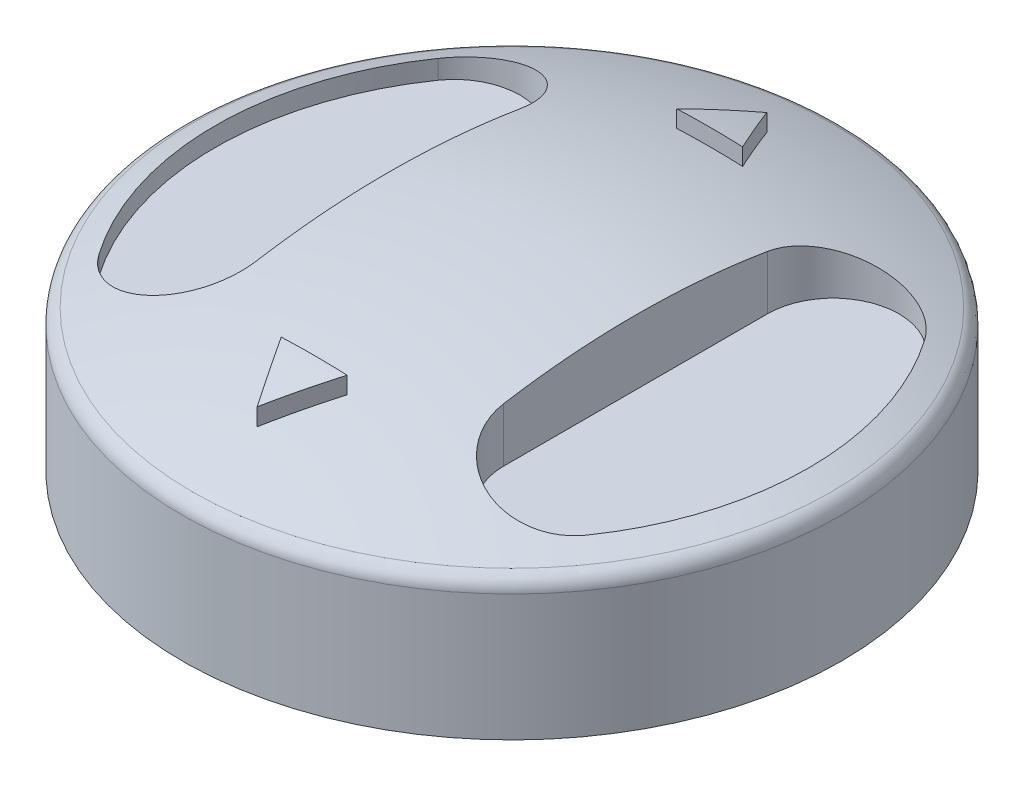
from build123d import *

# Parameters (mm, degrees)
FILLET1_R           = 1
SKETCH2_R           = 10
BOSS_EXTRUDE1_DEPTH = 2.5
CUT_EXTRUDE1_DEPTH  = 10.5
BOSS_EXTRUDE2_DEPTH = 13.5


with BuildPart() as part:
    # Sketch1 → Revolve1 (revolve)
    with BuildSketch(Plane.XY):
        with BuildLine():
            Line((20, 8.32575695), (20, 0))
            Line((20, 0), (0, 0))
            Line((0, 0), (0, 12.5))
            ThreePointArc((0, 12.5), (10.215482184, 11.445315647), (20, 8.32575695))
        make_face()
    revolve(axis=Axis((0, 0, 0), (0, 1, 0)))

    # Fillet1
    fillet1_edges = [part.edges().sort_by_distance(p)[0] for p in [
        (-20, 8.32575695, 0),
    ]]
    fillet(fillet1_edges, radius=FILLET1_R)

    # Sketch2 → Boss-Extrude1 (add)
    with BuildSketch(Plane.XZ):
        Circle(SKETCH2_R)
    extrude(amount=BOSS_EXTRUDE1_DEPTH)

    # Sketch3 → Cut-Extrude1 (cut)
    with BuildSketch(Plane(origin=(0, 8, 0), x_dir=(-1, 0, 0), z_dir=(0, -1, 0))):
        with BuildLine():
            Line((7.5, 8), (7.5, -8))
            ThreePointArc((7.5, -8), (10.299205094, -11.811908762), (14.774238712, -10.282114106))
            ThreePointArc((14.774238712, -10.282114106), (18, 0), (14.774238712, 10.282114106))
            ThreePointArc((14.774238712, 10.282114106), (10.299205094, 11.811908762), (7.5, 8))
        make_face()
        with BuildLine():
            Line((-7.5, 8), (-7.5, -8))
            ThreePointArc((-7.5, -8), (-10.299205094, -11.811908762), (-14.774238712, -10.282114106))
            ThreePointArc((-14.774238712, -10.282114106), (-18, 0), (-14.774238712, 10.282114106))
            ThreePointArc((-14.774238712, 10.282114106), (-10.299205094, 11.811908762), (-7.5, 8))
        make_face()
    extrude(amount=-CUT_EXTRUDE1_DEPTH, mode=Mode.SUBTRACT)

    # Sketch5 → Boss-Extrude2 (add)
    with BuildSketch(Plane.XZ):
        Polygon((2, -12), (0, -15.464101615), (-2, -12), align=None)
        Polygon((2, 12), (0, 15.464101615), (-2, 12), align=None)
    extrude(amount=-BOSS_EXTRUDE2_DEPTH)

    # Sketch4 → Cut-Revolve3 (revolve, cut)
    with BuildSketch(Plane(origin=(0, 0, 0), x_dir=(0, 0, -1), z_dir=(1, 0, 0)), mode=Mode.PRIVATE) as cut_revolve3_sk:
        with BuildLine():
            Line((0, 17.5), (0, 13.5))
            ThreePointArc((0, 13.5), (9.805586606, 12.548481209), (19.245283019, 9.729430248))
            ThreePointArc((19.245283019, 9.729430248), (21.85213452, 10.826847786), (20.754716981, 13.433699287))
            ThreePointArc((20.754716981, 13.433699287), (10.574652222, 16.473852284), (0, 17.5))
        make_face()
    revolve(cut_revolve3_sk.sketch.rotate(Axis((0, 0, 0), (0, 1, 0)), 270), axis=Axis((0, 0, 0), (0, 1, 0)), mode=Mode.SUBTRACT)


solid = part.part
